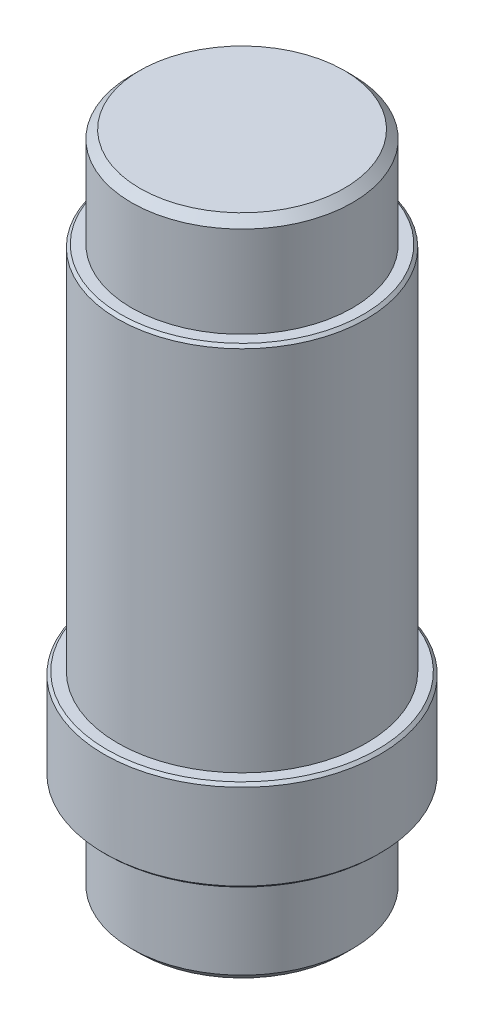
from build123d import *

# Parameters (mm, degrees)
SKETCH1_R           = 50
BOSS_EXTRUDE1_DEPTH = 120
SKETCH2_R           = 50
SKETCH2_R_2         = 40
CUT_EXTRUDE1_DEPTH  = 36
CUT_EXTRUDE2_START  = -37
SKETCH3_R           = 50
SKETCH3_R_2         = 40
CUT_EXTRUDE2_DEPTH  = 37
SKETCH4_R           = 50
SKETCH4_R_2         = 45
CUT_EXTRUDE3_DEPTH  = 134
CHAMFER1_SIZE       = 3
CHAMFER2_SIZE       = 1


with BuildPart() as part:
    # Sketch1 → Boss-Extrude1 (new, symmetric)
    with BuildSketch(Plane(origin=(0, 0, 0), x_dir=(1, 0, 0), z_dir=(0, 1, 0))):
        with Locations(Location((0, 0, 0), (0, 0, 270))):
            Circle(SKETCH1_R)
    extrude(amount=BOSS_EXTRUDE1_DEPTH, both=True)

    # Sketch2 → Cut-Extrude1 (cut)
    with BuildSketch(Plane(origin=(0, 120, 0), x_dir=(1, 0, 0), z_dir=(0, 1, 0))):
        with Locations(Location((0, 0, 0), (0, 0, 270))):
            Circle(SKETCH2_R)
        with Locations(Location((0, 0, 0), (0, 0, 270))):
            Circle(SKETCH2_R_2, mode=Mode.SUBTRACT)
    extrude(amount=-CUT_EXTRUDE1_DEPTH, mode=Mode.SUBTRACT)

    # Sketch3 → Cut-Extrude2 (cut)
    with BuildSketch(Plane.XZ.offset(120).offset(CUT_EXTRUDE2_START)):
        with Locations(Location((0, 0, 0), (0, 0, 270))):
            Circle(SKETCH3_R)
        with Locations(Location((0, 0, 0), (0, 0, 90))):
            Circle(SKETCH3_R_2, mode=Mode.SUBTRACT)
    extrude(amount=CUT_EXTRUDE2_DEPTH, mode=Mode.SUBTRACT)

    # Sketch4 → Cut-Extrude3 (cut)
    with BuildSketch(Plane(origin=(0, 84, 0), x_dir=(1, 0, 0), z_dir=(0, 1, 0))):
        with Locations(Location((0, 0, 0), (0, 0, 90))):
            Circle(SKETCH4_R)
        with Locations(Location((0, 0, 0), (0, 0, 270))):
            Circle(SKETCH4_R_2, mode=Mode.SUBTRACT)
    extrude(amount=-CUT_EXTRUDE3_DEPTH, mode=Mode.SUBTRACT)

    # Chamfer1
    chamfer1_edges = [part.edges().sort_by_distance(p)[0] for p in [
        (0, -120, -40),
        (0, 120, -40),
    ]]
    chamfer(chamfer1_edges, length=CHAMFER1_SIZE)

    # Chamfer2
    chamfer2_edges = [part.edges().sort_by_distance(p)[0] for p in [
        (0, -83, -50),
        (0, -50, -50),
        (0, 84, -45),
    ]]
    chamfer(chamfer2_edges, length=CHAMFER2_SIZE)


solid = part.part
